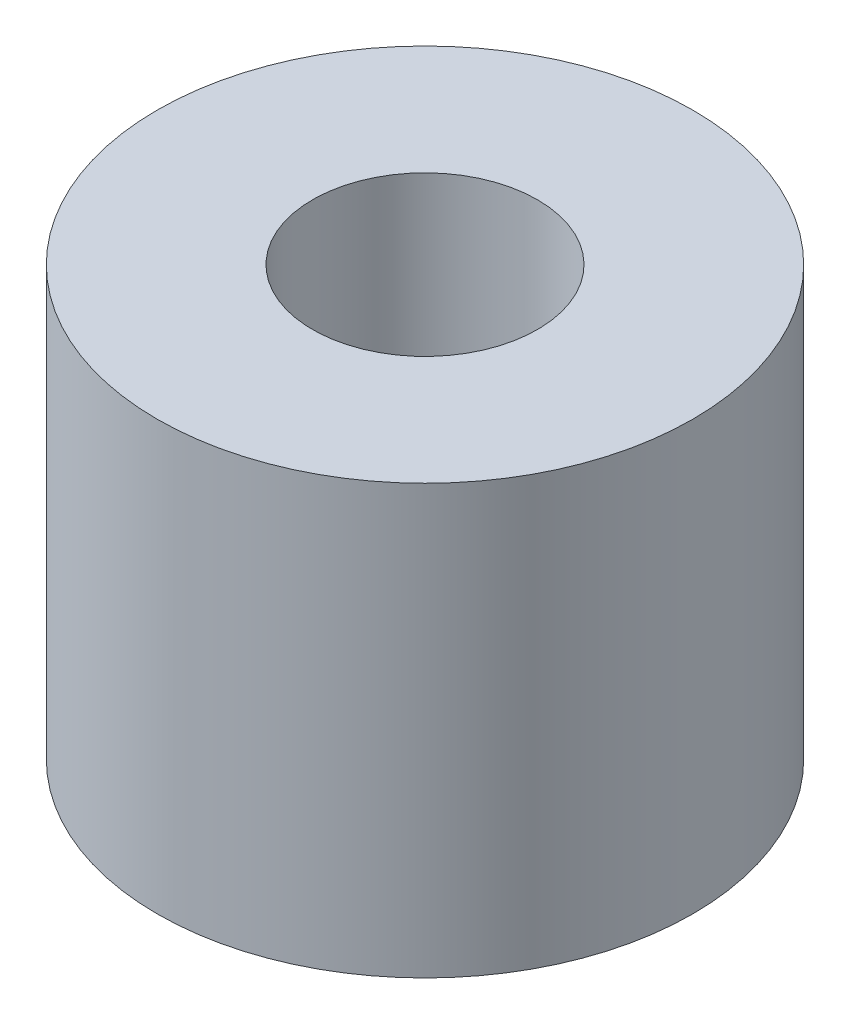
SolidWorks part; units mm, degrees
ref_plane "Front Plane" through (0, 0, 0) normal (0, 0, 1) x (1, 0, 0)
ref_plane "Top Plane" through (0, 0, 0) normal (0, 1, 0) x (1, 0, 0)
ref_plane "Right Plane" through (0, 0, 0) normal (1, 0, 0) x (0, 0, -1)
other "Configuration Table"
sketch "Sketch1" plane through (0, 0, 0) normal (0, 1, 0) x (1, 0, 0)
  circle A0 centre (0, 0) radius 25
  dimension "D1" = 50
extrude "Boss-Extrude1" add sketch "Sketch1" along normal blind 40
hole_wizard "M24 Tapped Hole1" positions "Sketch3" profile "Sketch4" tap size "M24" standard "GB" end condition through all
sketch "Sketch3" plane through (0, 0, 0) normal (0, -1, 0) x (-1, 0, 0)
  point P0 (0, 0)
sketch "Sketch4" plane through (0, 0, 0) normal (1, 0, 0) x (0, 0, -1)
  line L0 (0, 0) -> (0, 40)
  line L1 (0, 40) -> (10.5, 40)
  line L2 (10.5, 40) -> (10.5, 1.525)
  line L3 (10.5, 1.525) -> (12.025, 0)
  line L5 (12.025, 0) -> (0, 0)
  line L6 (-10.5, 1.525) -> (-12.025, 0) construction
  line L11 (0, -6.35) -> (0, 107.95) construction
  dimension "通孔螺纹孔钻头直径" = 21
  dimension "通孔螺纹孔钻头深度" = 40
  dimension "近端锥形沉头孔直径" = 24.05
  dimension "近端锥形沉头孔角度" = 90
cosmetic thread "Cosmetic Thread 1" parameters "D2"=24
